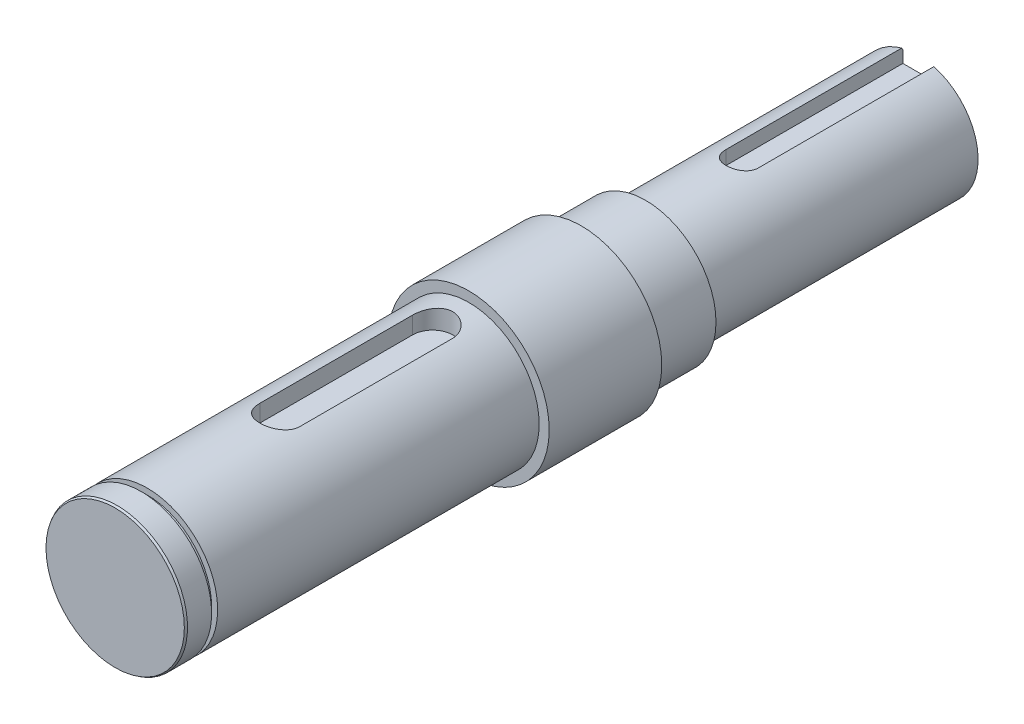
from build123d import *
from OCP.BRepFilletAPI import BRepFilletAPI_MakeChamfer

# Parameters (mm, degrees)
SKETCH1_R           = 15
BOSS_EXTRUDE1_DEPTH = 68
SKETCH2_R           = 17.5
BOSS_EXTRUDE2_DEPTH = 16
SKETCH3_R           = 20
BOSS_EXTRUDE3_DEPTH = 28
SKETCH4_R           = 17.5
BOSS_EXTRUDE4_DEPTH = 80
SKETCH5_R           = 16
BOSS_EXTRUDE5_DEPTH = 1.5
SKETCH6_R           = 17.5
BOSS_EXTRUDE6_DEPTH = 6.5
CUT_EXTRUDE1_START  = 17.5
CUT_EXTRUDE1_DEPTH  = 5
CUT_EXTRUDE2_START  = 15
CUT_EXTRUDE2_DEPTH  = 4
CUT_EXTRUDE3_START  = -15
CUT_EXTRUDE3_DEPTH  = 4
CHAMFER1_SIZE       = 0.5
CHAMFER1_SIZE2      = 0.288675135


with BuildPart() as part:
    # Sketch1 → Boss-Extrude1 (new body)
    with BuildSketch(Plane.XY):
        Circle(SKETCH1_R)
    extrude(amount=BOSS_EXTRUDE1_DEPTH)

    # Sketch2 → Boss-Extrude2 (add)
    with BuildSketch(Plane.XY.offset(68)):
        Circle(SKETCH2_R)
    extrude(amount=BOSS_EXTRUDE2_DEPTH)

    # Sketch3 → Boss-Extrude3 (add)
    with BuildSketch(Plane.XY.offset(84)):
        Circle(SKETCH3_R)
    extrude(amount=BOSS_EXTRUDE3_DEPTH)

    # Sketch4 → Boss-Extrude4 (add)
    with BuildSketch(Plane.XY.offset(112)):
        Circle(SKETCH4_R)
    extrude(amount=BOSS_EXTRUDE4_DEPTH)

    # Sketch5 → Boss-Extrude5 (add)
    with BuildSketch(Plane.XY.offset(192)):
        Circle(SKETCH5_R)
    extrude(amount=BOSS_EXTRUDE5_DEPTH)

    # Sketch6 → Boss-Extrude6 (add)
    with BuildSketch(Plane.XY.offset(193.5)):
        Circle(SKETCH6_R)
    extrude(amount=BOSS_EXTRUDE6_DEPTH)

    # Sketch7 → Cut-Extrude1 (cut)
    with BuildSketch(Plane(origin=(0, 0, 0), x_dir=(1, 0, 0), z_dir=(0, 1, 0)).offset(CUT_EXTRUDE1_START)):
        with BuildLine():
            Line((-5, -159), (-5, -121))
            ThreePointArc((-5, -121), (0, -116), (5, -121))
            Line((5, -121), (5, -159))
            ThreePointArc((5, -159), (0, -164), (-5, -159))
        make_face()
    extrude(amount=-CUT_EXTRUDE1_DEPTH, mode=Mode.SUBTRACT)

    # Sketch8 → Cut-Extrude2 (cut)
    with BuildSketch(Plane(origin=(0, 0, 0), x_dir=(1, 0, 0), z_dir=(0, 1, 0)).offset(CUT_EXTRUDE2_START)):
        with BuildLine():
            Line((-4, -44), (-4, 0))
            ThreePointArc((-4, 0), (0, 4), (4, 0))
            Line((4, 0), (4, -44))
            ThreePointArc((4, -44), (0, -48), (-4, -44))
        make_face()
    extrude(amount=-CUT_EXTRUDE2_DEPTH, mode=Mode.SUBTRACT)

    # Sketch9 → Cut-Extrude3 (cut)
    with BuildSketch(Plane(origin=(0, 0, 0), x_dir=(1, 0, 0), z_dir=(0, 1, 0)).offset(CUT_EXTRUDE3_START)):
        with BuildLine():
            Line((-4, -61), (-4, -54))
            ThreePointArc((-4, -54), (0, -50), (4, -54))
            Line((4, -54), (4, -61))
            ThreePointArc((4, -61), (0, -65), (-4, -61))
        make_face()
    extrude(amount=CUT_EXTRUDE3_DEPTH, mode=Mode.SUBTRACT)

    # Chamfer1: one chamfer whose edges measure the first distance from different faces: ONE call of the kernel's chamfer builder (chamfer() names one face for all edges)
    chamfer1_edges_1 = [part.edges().sort_by_distance(p)[0] for p in [
        (-17.5, 0, 200),
    ]]
    chamfer1_side_1 = [part.faces().sort_by_distance(p)[0] for p in [
        (-17.5, 0, 196.75),
    ]]
    chamfer1_edges_2 = [part.edges().sort_by_distance(p)[0] for p in [
        (-9.082951062, -11.937336386, 0),
    ]]
    chamfer1_side_2 = [part.faces().sort_by_distance(p)[0] for p in [
        (0, -0.583570782, 0),
    ]]
    chamfer1 = BRepFilletAPI_MakeChamfer(part.part.solid().wrapped)
    for e in chamfer1_edges_1:
        chamfer1.Add(CHAMFER1_SIZE, CHAMFER1_SIZE2, e.wrapped, chamfer1_side_1[0].wrapped)  # the first distance lies on this face
    for e in chamfer1_edges_2:
        chamfer1.Add(CHAMFER1_SIZE, CHAMFER1_SIZE2, e.wrapped, chamfer1_side_2[0].wrapped)  # the first distance lies on this face
    add(Compound.cast(chamfer1.Shape()), mode=Mode.REPLACE)


solid = part.part
